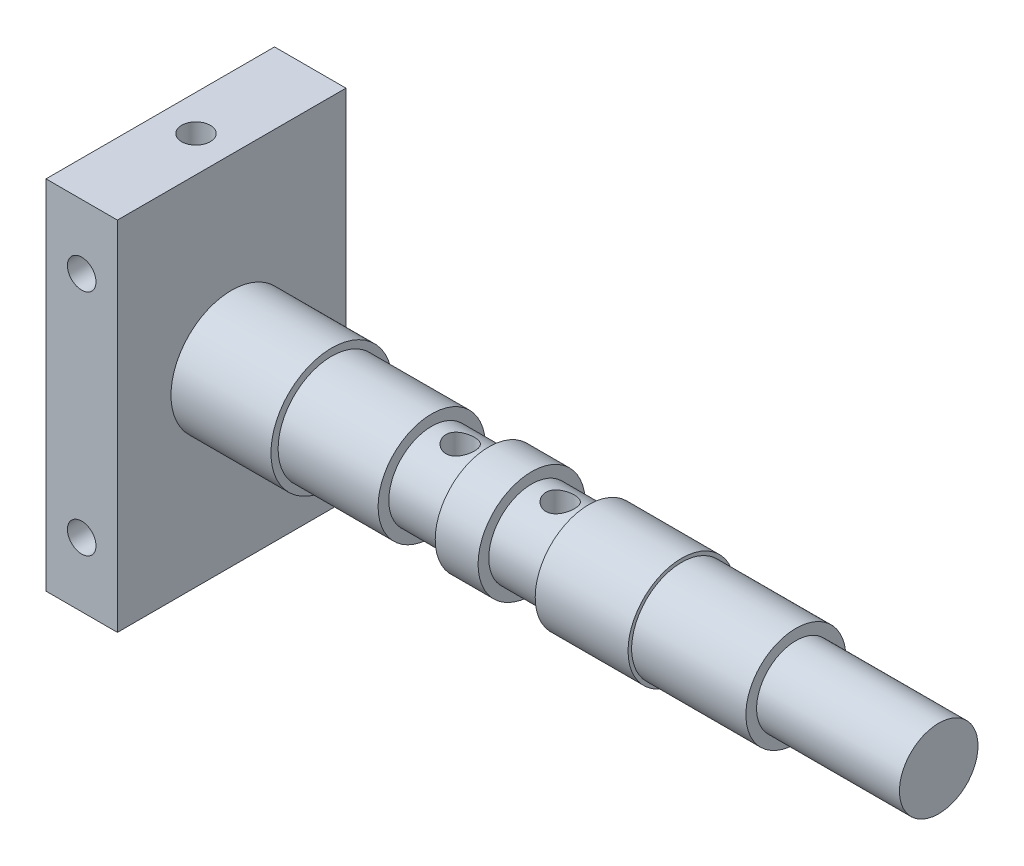
SolidWorks part; units mm, degrees
ref_plane "Front Plane" through (0, 0, 0) normal (0, 0, 1) x (1, 0, 0)
ref_plane "Top Plane" through (0, 0, 0) normal (0, 1, 0) x (1, 0, 0)
ref_plane "Right Plane" through (0, 0, 0) normal (1, 0, 0) x (0, 0, -1)
sketch "Sketch1" plane through (0, 0, 0) normal (1, 0, 0) x (0, 0, -1)
  line L1 (-16, 25) -> (16, 25)
  line L2 (-16, 25) -> (-16, -25)
  line L3 (-16, -25) -> (16, -25)
  line L4 (16, 25) -> (16, -25)
  line L5 (-16, 25) -> (16, -25) construction
  line L6 (-16, -25) -> (16, 25) construction
  point P0 (0, 0)
  dimension "D1" = 50
  dimension "D2" = 32
extrude "Boss-Extrude1" add sketch "Sketch1" along normal blind 10
sketch "Sketch2" plane through (10, 0, 0) normal (1, 0, 0) x (0, 0, -1)
  circle A0 centre (0, 0) radius 8.5
  dimension "D1" = 17
extrude "Boss-Extrude2" add sketch "Sketch2" along normal blind 14
sketch "Sketch3" plane through (0, 0, 16) normal (0, 0, 1) x (1, 0, 0)
  line L0 (0, 0) -> (29.0325, 0) construction
  line L1 (0, 25) -> (0, -25) construction
  circle A0 centre (5, 16) radius 2
  circle A1 centre (5, -16) radius 2
  dimension "D2" = 4
  dimension "D1" = 32
  dimension "D3" = 5
extrude "Cut-Extrude1" cut sketch "Sketch3" against normal blind 24
sketch "Sketch4" plane through (0, 25, 0) normal (0, 1, 0) x (1, 0, 0)
  circle A0 centre (5, 0) radius 2
  dimension "D2" = 4
  dimension "D1" = 5
extrude "Cut-Extrude2" cut sketch "Sketch4" against normal blind 45
sketch "Sketch5" plane through (24, 0, 0) normal (1, 0, 0) x (0, 0, -1)
  circle A0 centre (0, 0) radius 7.5
  dimension "D1" = 15
extrude "Boss-Extrude3" add sketch "Sketch5" along normal blind 65
sketch "Sketch6" plane through (0, 0, 0) normal (0, 0, 1) x (1, 0, 0)
  line L0 (0, 0) -> (136.7914, 0) construction
  line L1 (89, 7.5) -> (24, 7.5) construction
  line L2 (38, 7.5) -> (46, 7.5)
  line L3 (38, 7.5) -> (38, 6)
  line L4 (38, 6) -> (46, 6)
  line L5 (46, 7.5) -> (46, 6)
  line L7 (52, 7.5) -> (60, 7.5)
  line L8 (52, 7.5) -> (52, 6)
  line L9 (52, 6) -> (60, 6)
  line L10 (60, 7.5) -> (60, 6)
  dimension "D1" = 8
  dimension "D2" = 1.5
  dimension "D3" = 38
  dimension "D4" = 14
revolve "Cut-Revolve1" cut sketch "Sketch6" angle 360 about L0
sketch "Sketch7" plane through (89, 0, 0) normal (1, 0, 0) x (0, 0, -1)
  circle A0 centre (0, 0) radius 5.5
  dimension "D1" = 11
extrude "Boss-Extrude4" add sketch "Sketch7" along normal blind 20
ref_axis "Axis1" through (89, 0, 0) along (-1, 0, 0)
sketch "Sketch9" plane through (0, 0, 0) normal (0, 0, 1) x (1, 0, 0)
  line L0 (89, -7.5) -> (89, 7.5) construction
  line L1 (89, 7.5) -> (73, 7.5)
  line L2 (89, 7.5) -> (89, 7)
  line L3 (89, 7) -> (73, 7)
  line L4 (73, 7.5) -> (73, 7)
  line L5 (89, 7.5) -> (60, 7.5) construction
  dimension "D1" = 0.5
  dimension "D2" = 16
revolve "Cut-Revolve2" cut sketch "Sketch9" angle 360 about axis through (89, 0, 0) along (-1, 0, 0)
sketch "Sketch10" plane through (0, 0, 0) normal (-1, 0, 0) x (0, 0, 1)
  circle A0 centre (0, 0) radius 2.5
  dimension "D1" = 5
extrude "Cut-Extrude3" cut sketch "Sketch10" against normal blind 66
sketch "Sketch11" plane through (0, 25, 0) normal (0, 1, 0) x (1, 0, 0)
  circle A0 centre (42, 0) radius 2
  circle A1 centre (56, 0) radius 2
  dimension "D3" = 4
  dimension "D1" = 42
  dimension "D2" = 56
extrude "Cut-Extrude4" cut sketch "Sketch11" against normal blind 24
